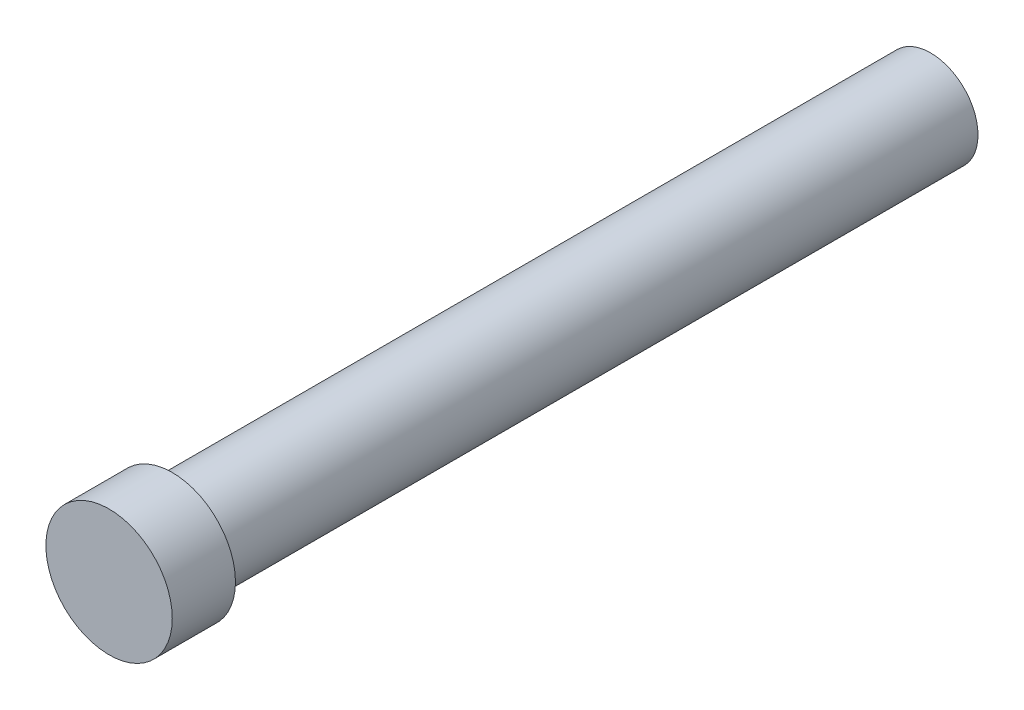
SolidWorks part; units mm, degrees
ref_plane "前视基准面" through (0, 0, 0) normal (0, 0, 1) x (1, 0, 0)
ref_plane "上视基准面" through (0, 0, 0) normal (0, 1, 0) x (1, 0, 0)
ref_plane "右视基准面" through (0, 0, 0) normal (1, 0, 0) x (0, 0, -1)
sketch "草图1" plane through (0, 0, 0) normal (0, 0, 1) x (1, 0, 0)
  circle A0 centre (0, 0) radius 0.75
  dimension "D1" = 1.5
extrude "凸台-拉伸1" add sketch "草图1" along normal blind 12
sketch "草图2" plane through (0, 0, 12) normal (0, 0, 1) x (1, 0, 0)
  circle A0 centre (0, 0) radius 1
  dimension "D1" = 2
extrude "凸台-拉伸2" add sketch "草图2" along normal blind 1
